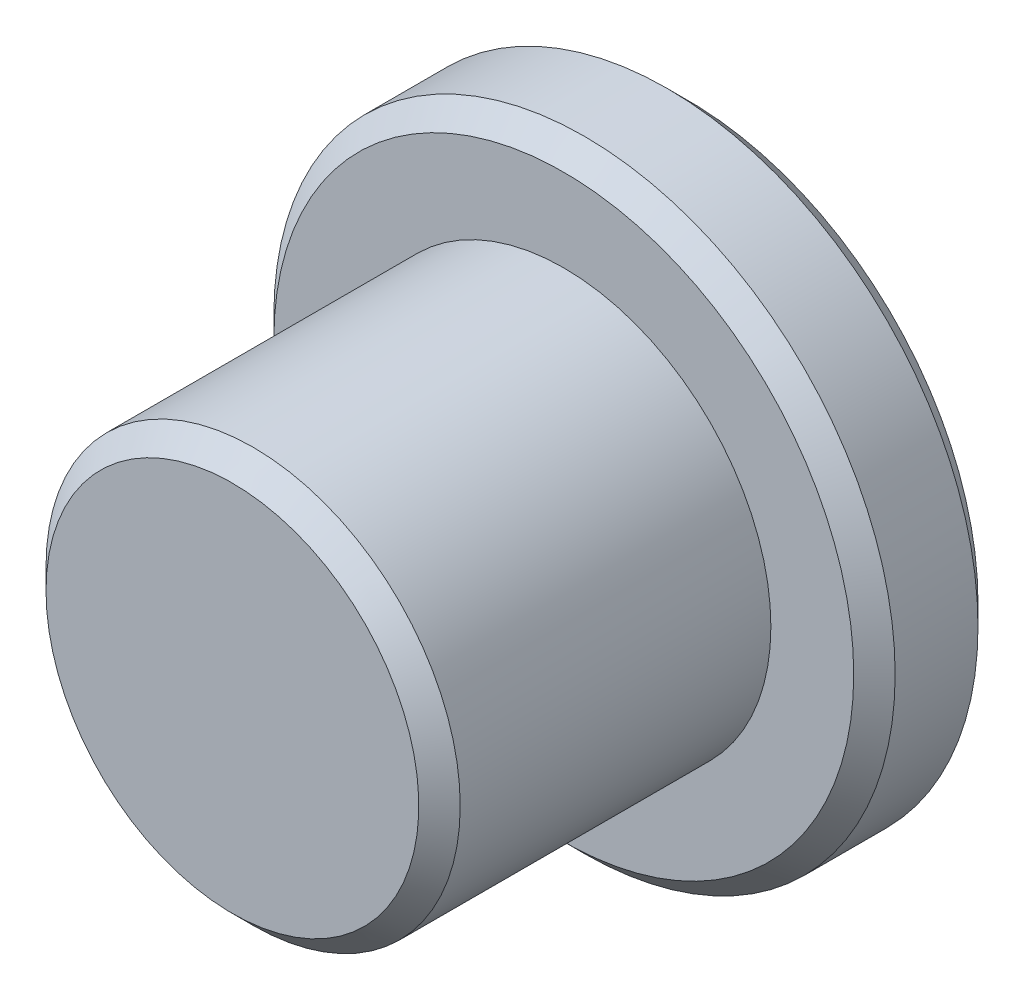
SolidWorks part; units mm, degrees
material "Q235B"
ref_plane "Front Plane" through (0, 0, 0) normal (0, 0, 1) x (1, 0, 0)
ref_plane "Top Plane" through (0, 0, 0) normal (0, 1, 0) x (1, 0, 0)
ref_plane "Right Plane" through (0, 0, 0) normal (1, 0, 0) x (0, 0, -1)
sketch "Sketch1" plane through (0, 0, 0) normal (1, 0, 0) x (0, 0, -1)
  line L0 (0, 0) -> (11, 0) construction
  line L1 (11, 0) -> (11, 7.5)
  line L2 (11, 7.5) -> (8, 7.5)
  line L3 (8, 7.5) -> (8, 5)
  line L4 (8, 5) -> (0, 5)
  line L5 (0, 5) -> (0, 0)
  line L6 (0, 0) -> (11, 0)
  dimension "D1" = 5
  dimension "D2" = 7.5
  dimension "D3" = 3
  dimension "D4" = 8
revolve "Revolve1" add sketch "Sketch1" angle 360 about L0
chamfer "Chamfer1" distance 0.5 angle 45 3 edges at (7.5, 0, -11) (7.5, 0, -8) (5, 0, 0)
